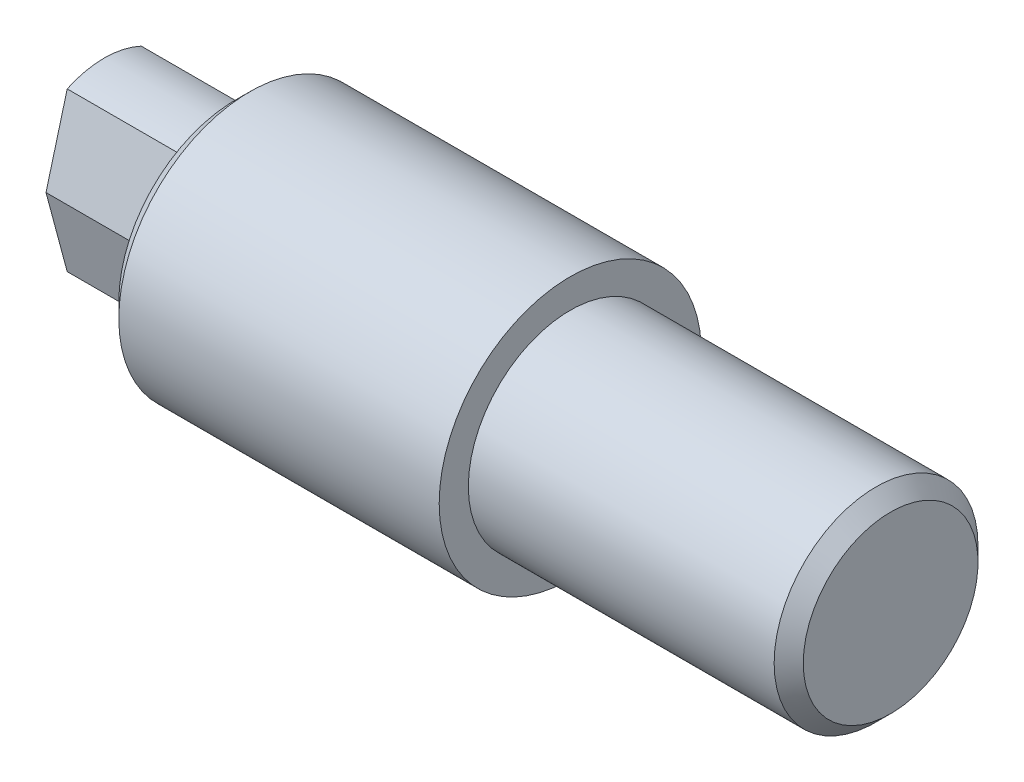
SolidWorks part; units mm, degrees
ref_plane "Front Plane" through (0, 0, 0) normal (0, 0, 1) x (1, 0, 0)
ref_plane "Top Plane" through (0, 0, 0) normal (0, 1, 0) x (1, 0, 0)
ref_plane "Right Plane" through (0, 0, 0) normal (1, 0, 0) x (0, 0, -1)
sketch "Sketch1" plane through (0, 0, 0) normal (0, 0, 1) x (1, 0, 0)
  line L0 (-65.3189, 0) -> (82.7141, 0) construction
  line L1 (-21.4727, 0) -> (-21.4727, 9)
  line L2 (-21.4727, 9) -> (1.5273, 9)
  line L3 (1.5273, 9) -> (1.5273, 7)
  line L4 (1.5273, 7) -> (23.5273, 7)
  line L5 (23.5273, 7) -> (23.5273, 0)
  line L6 (23.5273, 0) -> (-21.4727, 0)
  dimension "D1" = 23
  dimension "D2" = 22
  dimension "D3" = 7
  dimension "D4" = 9
revolve "Revolve1" add sketch "Sketch1" angle 360 about L0
chamfer "Chamfer1" distance 1 angle 45 1 edges at (23.5273, 0, 7)
chamfer "Chamfer2" distance 1 angle 45 1 edges at (-21.4727, 0, 9)
sketch "Sketch3" plane through (-21.4727, 0, 0) normal (-1, 0, 0) x (0, 0, 1)
  line L3 (4, 0) -> (2.544, 5.434)
  line L4 (-4, 0) -> (-2.544, 5.434)
  line L5 (-4, 0) -> (-2.544, -5.434)
  line L6 (4, 0) -> (2.544, -5.434)
  arc A0 (-2.544, -5.434) -> (2.544, -5.434) centre (0, 0) ccw
  arc A1 (2.544, 5.434) -> (-2.544, 5.434) centre (0, 0) ccw
  dimension "D1" = 12
extrude "Boss-Extrude1" add sketch "Sketch3" along normal blind 9
